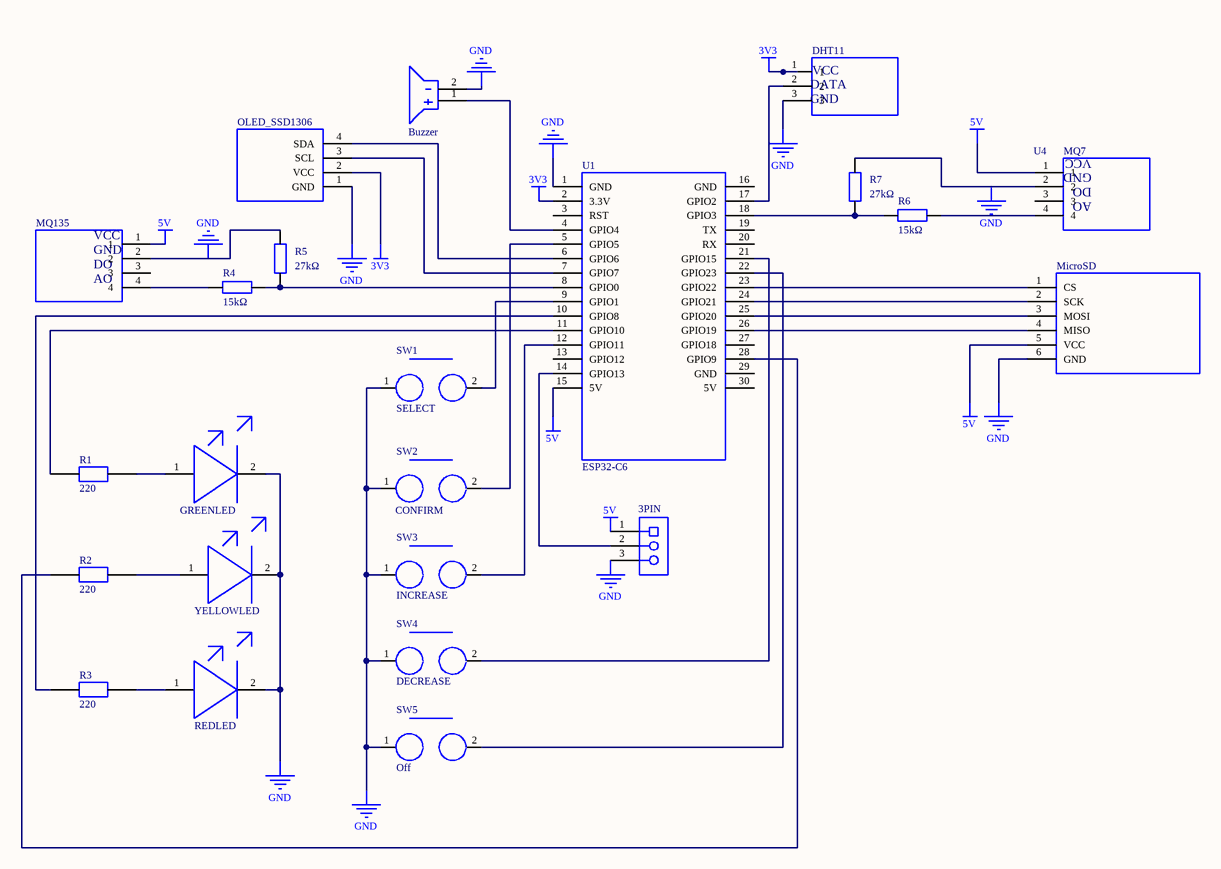
[diagram p0: MISC51777-3.schdoc]
# Altium project MISC51777-2.PrjPcb
1 sheet, 23 parts. Net scope: global (net labels, ports and power ports of the same name join across sheets).
Board file: MISC51777.pcbdoc

## Sheet MISC51777-3.schdoc
size 292 x 193 mm; SheetNumber: 1; SheetTotal: 1; @Page No: 1; @Page Count: 1; @Schematic Name: MISC51777; @Project Name: MISC51777; @Board Name: MISC51777; @Update Date: 2025-06-22; @Create Time: 21:02:52; @Update Time: 22:04:01; @Create Date: 2025-06-22

### Parts
3PIN  (no value)  [HDR-TH_3P-P2.54-V-F]
*  DHT11  [HDR-TH_3P-P2.54-V-F]
Buzzer1  Buzzer  [BUZ-TH_BD12.0-P6.00-D0.9-RD]
GREENLED  LED_3M  [LED_TH-3mm]  (value not drawn)
R1  220  [Res_1/8W]
R2  220  [Res_1/8W]
R3  220  [Res_1/8W]
R4  15kΩ  [Res_1/8W]
R5  27kΩ  [Res_1/8W]
R6  15kΩ  [Res_1/8W]
R7  27kΩ  [Res_1/8W]
REDLED  LED_3M  [LED_TH-3mm]  (value not drawn)
SW1  SELECT  [KEY-TH_2P-L6.0-W6.0-P5.00]
SW2  CONFIRM  [KEY-TH_2P-L6.0-W6.0-P5.00]
SW3  INCREASE  [KEY-TH_2P-L6.0-W6.0-P5.00]
SW4  DECREASE  [KEY-TH_2P-L6.0-W6.0-P5.00]
SW5  Off  [KEY-TH_2P-L6.0-W6.0-P5.00]
U1  ESP32-C6  [HDR-TH_33P-P2.54-V-R2-C15-S2.54_C9041]
U2  MicroSD  [HDR-TH_6P-P2.54-V-F]
U3  OLED_SSD1306  [0.96OLED_4P]
U4  MQ7  [HDR-TH_4P-P2.54-V-F]
U5  MQ135  [HDR-TH_4P-P2.54-V-F]
YELLOWLED  LED_3M  [LED_TH-3mm]  (value not drawn)

### Nets
3V3: *.1 U1.2(3.3V) U3.2(VCC)
5V: 3PIN.1 U1.15(5V) U2.5(VCC) U4.1 U5.1
GND: 3PIN.3 *.3 Buzzer1.2 GREENLED.2 R5.2 R7.2 REDLED.2 SW1.1 SW2.1 SW3.1 SW4.1 SW5.1 U1.1(GND) U2.6(GND) U3.1(GND) U4.2 U5.2 YELLOWLED.2
Net3PIN_2: 3PIN.2 U1.14(GPIO13)
Net*_2: *.2 U1.17(GPIO2)
NetBuzzer1_1: Buzzer1.1 U1.4(GPIO4)
NetGREENLED_1: GREENLED.1 R1.2
NetR1_1: R1.1 U1.11(GPIO10)
NetR2_1: R2.1 U1.28(GPIO9)
NetR2_2: R2.2 YELLOWLED.1
NetR3_1: R3.1 U1.10(GPIO8)
NetR3_2: R3.2 REDLED.1
NetR4_1: R4.1 U5.4
NetR4_2: R4.2 R5.1 U1.8(GPIO0)
NetR6_1: R6.1 R7.1 U1.18(GPIO3)
NetR6_2: R6.2 U4.4
NetSW1_2: SW1.2 U1.9(GPIO1)
NetSW2_2: SW2.2 U1.5(GPIO5)
NetSW3_2: SW3.2 U1.12(GPIO11)
NetSW4_2: SW4.2 U1.21(GPIO15)
NetSW5_2: SW5.2 U1.22(GPIO23)
NetU1_6: U1.6(GPIO6) U3.4(SDA)
NetU1_7: U1.7(GPIO7) U3.3(SCL)
NetU1_23: U1.23(GPIO22) U2.1(CS)
NetU1_24: U1.24(GPIO21) U2.2(SCK)
NetU1_25: U1.25(GPIO20) U2.3(MOSI)
NetU1_26: U1.26(GPIO19) U2.4(MISO)

Not connected (* = marked no-connect by the designer): U1 3(RST) 13(GPIO12) 16(GND) 19(TX) 20(RX) 27(GPIO18) 29(GND) 30(5V); U4 3; U5 3

### Notes on the sheet
- Title
- File:
- Date:
- Size
- A4
- Number
- Drawn By:
- Sheet
- Of
- Revision

### Library data of the parts
3PIN = CN-1P-M-R3: Male Header, Pitch 2.5 mm, 1 x 3 Position, Height 6.1 mm, Tail Length 3.4 mm, -25 to 85 degC, RoHS, Bulk; Manufacturer: JST; Origin Footprint: JST-S3B-XH-A(LF)(SN)_V; AddInBom: yes; Device: CN-1P-M-R3; Symbol: CN-1P-M-R3; Design Item ID: CMP-002-00033-2; Library Name: Yuxin Wei; Package Description: Male Header, Pitch 2.5 mm, 1 x 3 Position, Height 6.1 mm, Tail Length 3.4 mm; Manufacturer URL: http://www.jst.com/home2.html; Datasheet URL: http://www.jst-mfg.com/product/pdf/eng/eXH.pdf; RoHS Compliant: Unknown; Connector Type: Header; Package Reference: S3B-XH-A(LF)(SN); Gender: Male; Case/Package: S3B-XH-A(LF)(SN); Mounting Technology: TH; Max Operating Temperature: 85°C; Min Operating Temperature: -25°C; Datasheet Version: May-16; ConvertToPcb: yes
* = DHT11: AddInBom: yes; Origin Footprint: DHT11; Device: DHT11; Symbol: DHT11; Design Item ID: DHT11; Library Name: MQ; ConvertToPcb: yes
Buzzer1 = Buzzer: AddInBom: yes; Origin Footprint: BUZZER; Device: Buzzer; Symbol: Buzzer; Design Item ID: Buzzer; Library Name: ESP32C6_DevBoard; ConvertToPcb: yes
GREENLED REDLED YELLOWLED = LED_3M: AddInBom: yes; Origin Footprint: LED_3M; Device: LED_3M; Symbol: LED_3M; Design Item ID: LED_3M; Library Name: Schlib1; ConvertToPcb: yes
R1-R3 = 220: Origin Footprint 1: AXIAL0.4; Symbol: Resistor; AddInBom: yes; Device: 220; Design Item ID: Resistor; Library Name: Resistor; Origin Footprint 2: resistor; Origin Footprint 3: AXIAL0.4; ConvertToPcb: yes
R4-R7 = Res_AXIAL-1/8W: ConvertToPcb: yes; SymbolName: 电阻; ModelId: b2b5ae7ae4c642178fe0039925c86a3f; ModelName: RES-TH_BD1.8-L3.2-P7.20-D0.4; ModelTransform: 282.86,66.88,253.09,0,0,0,0,0,-191; Device: Res_AXIAL-1/8W; AddInBom: yes; Supplier Footprint: 轴向引线; FootprintName: Res_1/8W
  R4 R6: Value: 15kΩ
  R5 R7: Value: 27kΩ
SW1 = SELECT: Origin Footprint: 6X6X6H_2P; Symbol: Component_1; AddInBom: yes; Device: SELECT; Design Item ID: Component_1; Library Name: Schlib1; ConvertToPcb: yes
SW2 = CONFIRM: Origin Footprint: 6X6X6H_2P; Symbol: Component_1; AddInBom: yes; Device: CONFIRM; Design Item ID: Component_1; Library Name: Schlib1; ConvertToPcb: yes
SW3 = INCREASE: Origin Footprint: 6X6X6H_2P; Symbol: Component_1; AddInBom: yes; Device: INCREASE; Design Item ID: Component_1; Library Name: Schlib1; ConvertToPcb: yes
SW4 = DECREASE: Origin Footprint: 6X6X6H_2P; Symbol: Component_1; AddInBom: yes; Device: DECREASE; Design Item ID: Component_1; Library Name: Schlib1; ConvertToPcb: yes
SW5 = Off: Origin Footprint: 6X6X6H_2P; Symbol: Component_1; AddInBom: yes; Device: Off; Design Item ID: Component_1; Library Name: Schlib1; ConvertToPcb: yes
U1 = ESP32-C6: Origin Footprint: 1.ESP32C6; AddInBom: yes; Device: ESP32-C6; Symbol: ESP32-C6; Design Item ID: ESP32-C6; Library Name: ESP32C6_DevBoard; ConvertToPcb: yes
U2 = MicroSD: Origin Footprint: SD; AddInBom: yes; Device: MicroSD; Symbol: MicroSD; Design Item ID: MicroSD; Library Name: SD; ConvertToPcb: yes
U3 = OLED_SSD1306: Origin Footprint 1: OLED; AddInBom: yes; Device: OLED_SSD1306; Symbol: OLED_SSD1306; Design Item ID: OLED_SSD1306; Library Name: ESP32C6_DevBoard; Origin Footprint 2: OLED; ConvertToPcb: yes
U4 = MQ7: AddInBom: yes; Origin Footprint: MQ7; Device: MQ7; Symbol: MQ7; Design Item ID: MQ7; Library Name: MQ; ConvertToPcb: yes
U5 = MQ135: Origin Footprint: MQ7; AddInBom: yes; Device: MQ135; Symbol: MQ7; Design Item ID: MQ7; Library Name: MQ; ConvertToPcb: yes